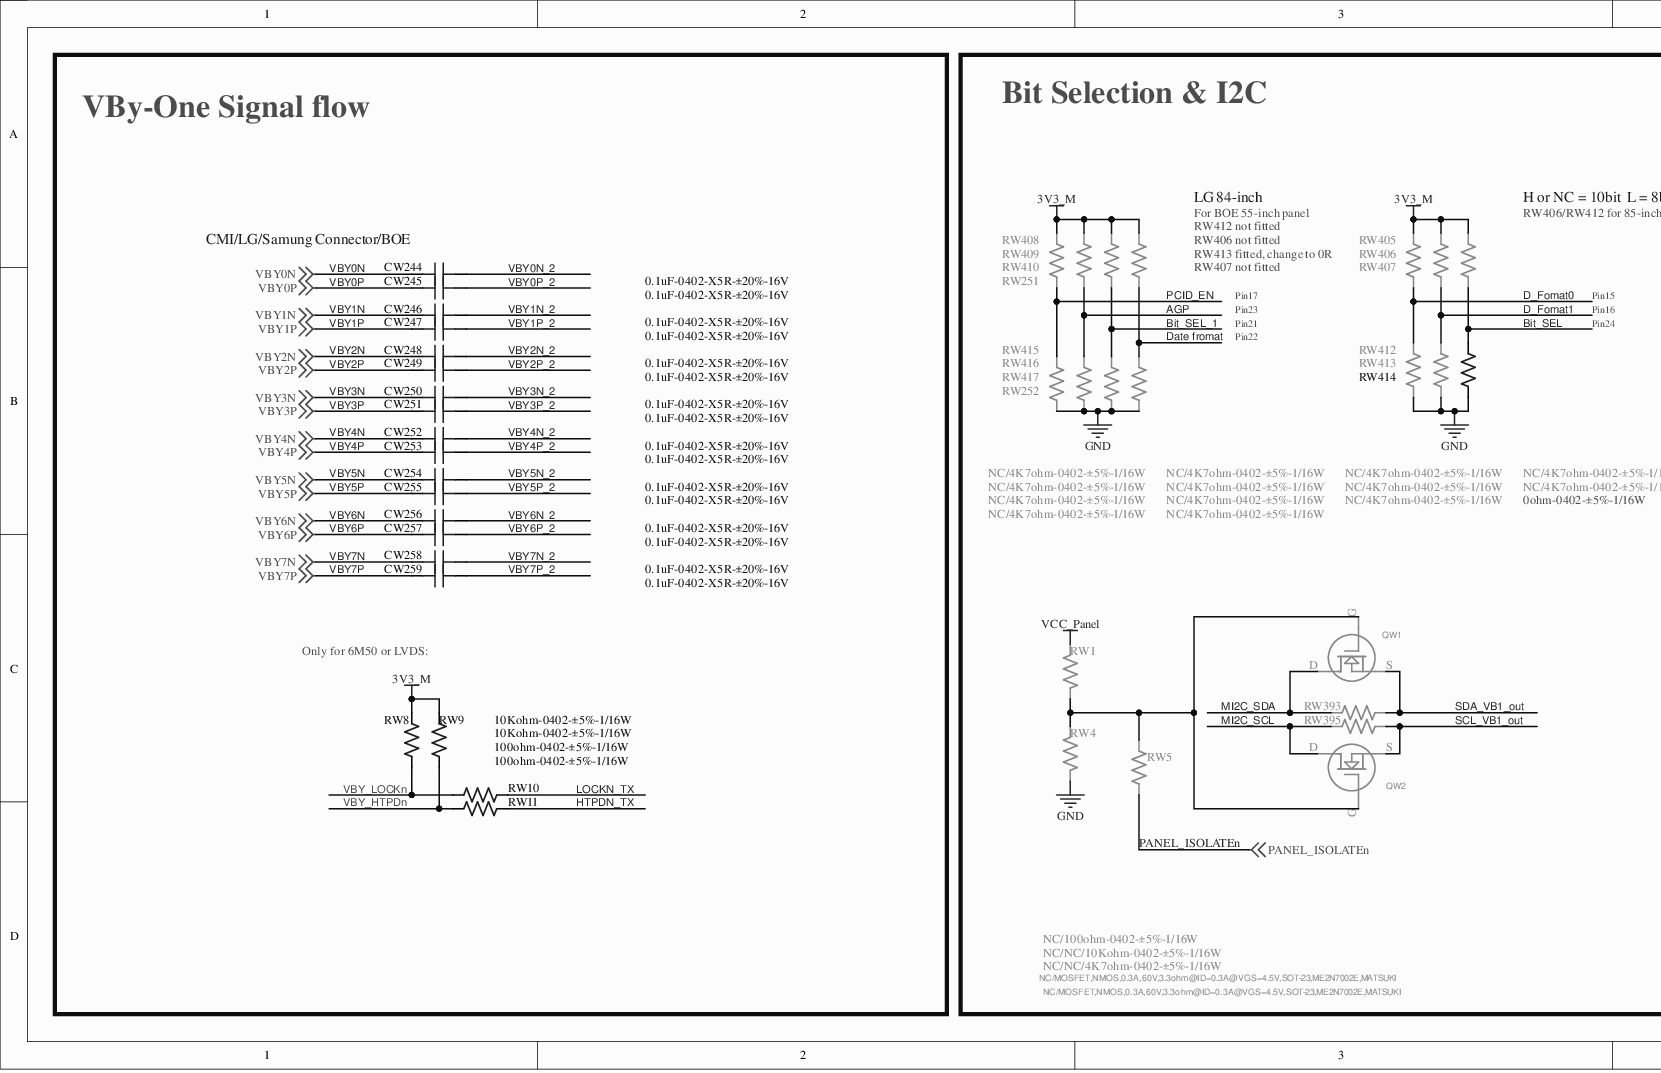
[diagram p0: MISC86290-12.SchDoc, left]
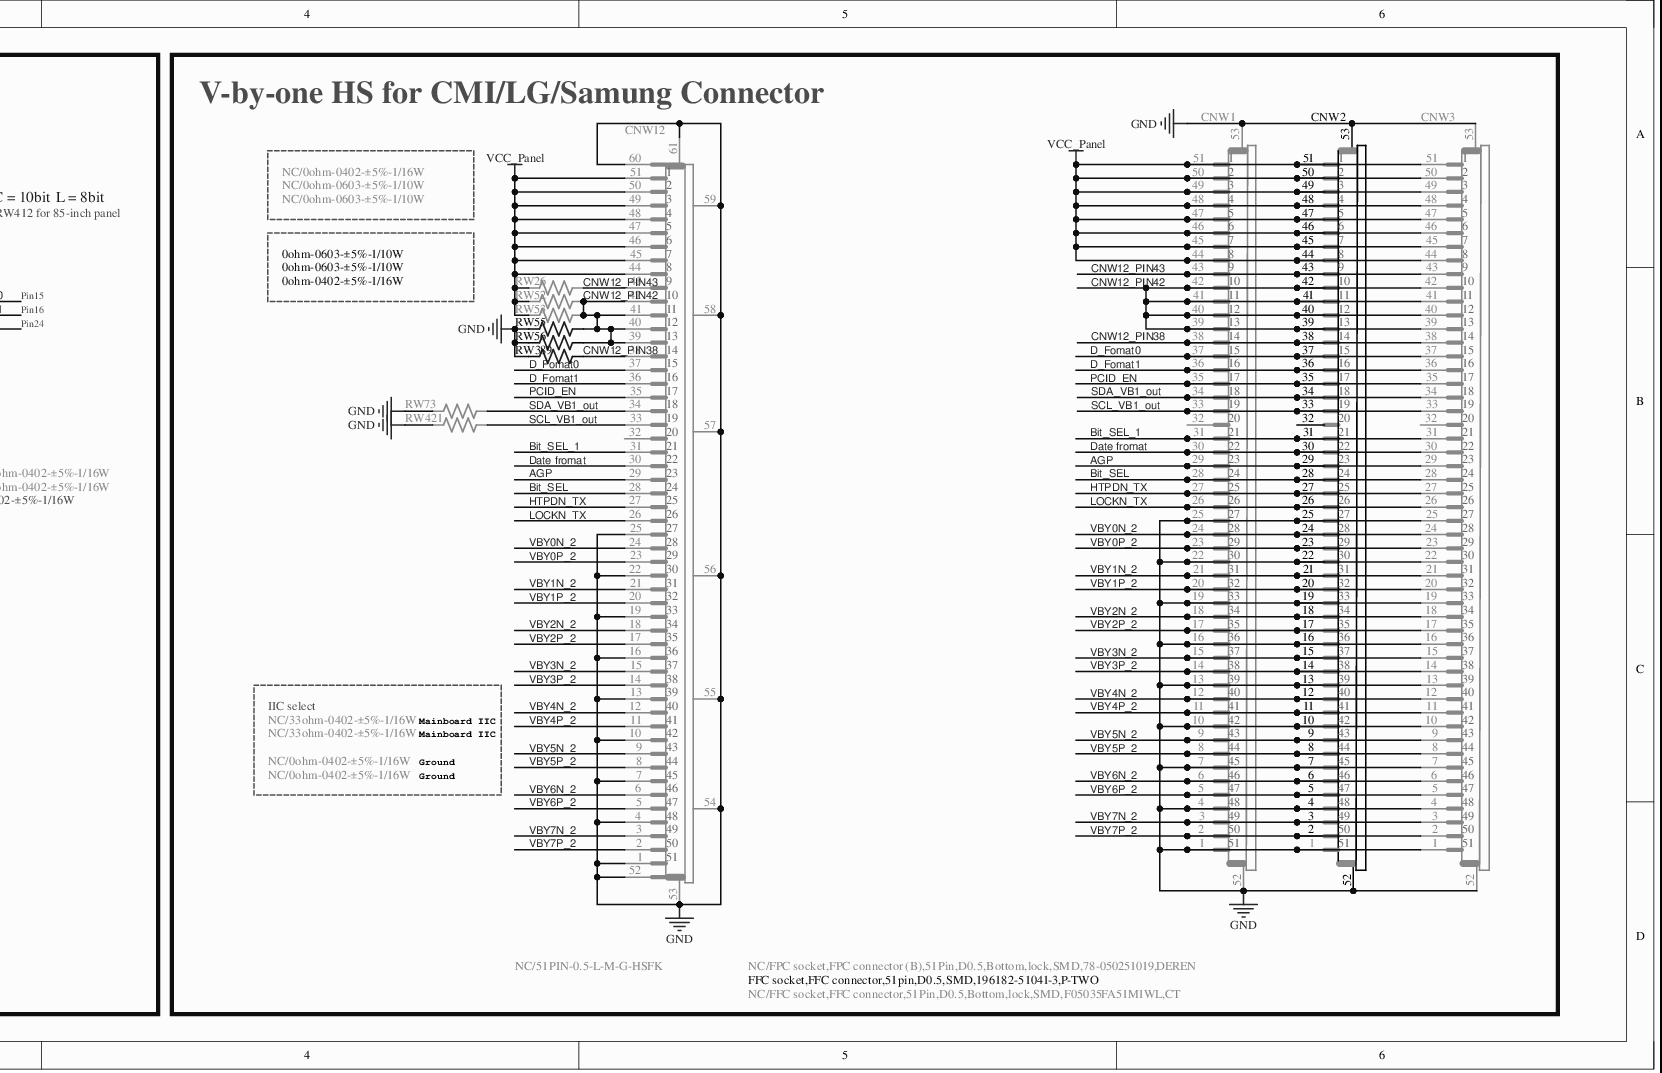
[diagram p1: MISC86290-12.SchDoc, right]
# Altium project MISC86290.PrjPcb (part 9 of 13)

## Sheet MISC86290-12.SchDoc
size 596 x 198 mm

### Parts
CNW1  NC/FPC socket,FPC connector (B),51Pin,D0.5,Bottom,lock,SMD,78-050251019,DEREN  [FFC51H/0.5S-10]
CNW2  FFC socket,FFC connector,51pin,D0.5,SMD,196182-51041-3,P-TWO  [FFC51-H/0.5S-1]
CNW3  NC/FFC socket,FFC connector,51Pin,D0.5,Bottom,lock,SMD,F05035FA51M1WL,CT  [FFC51H/0.5S-12]
CNW12  NC/51PIN-0.5-L-M-G-HSFK  [FFC51H/0.5SA-1]
CW244  0.1uF-0402-X5R-±20%-16V  [C0402]
CW245  0.1uF-0402-X5R-±20%-16V  [C0402]
CW246  0.1uF-0402-X5R-±20%-16V  [C0402]
CW247  0.1uF-0402-X5R-±20%-16V  [C0402]
CW248  0.1uF-0402-X5R-±20%-16V  [C0402]
CW249  0.1uF-0402-X5R-±20%-16V  [C0402]
CW250  0.1uF-0402-X5R-±20%-16V  [C0402]
CW251  0.1uF-0402-X5R-±20%-16V  [C0402]
CW252  0.1uF-0402-X5R-±20%-16V  [C0402]
CW253  0.1uF-0402-X5R-±20%-16V  [C0402]
CW254  0.1uF-0402-X5R-±20%-16V  [C0402]
CW255  0.1uF-0402-X5R-±20%-16V  [C0402]
CW256  0.1uF-0402-X5R-±20%-16V  [C0402]
CW257  0.1uF-0402-X5R-±20%-16V  [C0402]
CW258  0.1uF-0402-X5R-±20%-16V  [C0402]
CW259  0.1uF-0402-X5R-±20%-16V  [C0402]
QW1  NC/MOSFET,NMOS,0.3A,60V,3.3ohm@ID=0.3A@VGS=4.5V,SOT-23,ME2N7002E,MATSUKI  [SOT-23-7]
QW2  NC/MOSFET,NMOS,0.3A,60V,3.3ohm@ID=0.3A@VGS=4.5V,SOT-23,ME2N7002E,MATSUKI  [SOT-23-7]
RW1  NC/NC/10Kohm-0402-±5%-1/16W  [R0402]
RW4  NC/NC/4K7ohm-0402-±5%-1/16W  [R0402]
RW5  NC/100ohm-0402-±5%-1/16W  [R0402]
RW8  10Kohm-0402-±5%-1/16W  [R0402]
RW9  10Kohm-0402-±5%-1/16W  [R0402]
RW10  100ohm-0402-±5%-1/16W  [R0402]
RW11  100ohm-0402-±5%-1/16W  [R0402]
RW26  NC/0ohm-0402-±5%-1/16W  [R0402]
RW52  NC/0ohm-0603-±5%-1/10W  [R0603]
RW53  NC/0ohm-0603-±5%-1/10W  [R0603]
RW55  0ohm-0603-±5%-1/10W  [R0603]
RW56  0ohm-0603-±5%-1/10W  [R0603]
RW73  NC/0ohm-0402-±5%-1/16W  [R0402]
RW251  NC/4K7ohm-0402-±5%-1/16W  [R0402]
RW252  NC/4K7ohm-0402-±5%-1/16W  [R0402]
RW389  0ohm-0402-±5%-1/16W  [R0402]
RW393  NC/33ohm-0402-±5%-1/16W  [R0402]
RW395  NC/33ohm-0402-±5%-1/16W  [R0402]
RW405  NC/4K7ohm-0402-±5%-1/16W  [R0402]
RW406  NC/4K7ohm-0402-±5%-1/16W  [R0402]
RW407  NC/4K7ohm-0402-±5%-1/16W  [R0402]
RW408  NC/4K7ohm-0402-±5%-1/16W  [R0402]
RW409  NC/4K7ohm-0402-±5%-1/16W  [R0402]
RW410  NC/4K7ohm-0402-±5%-1/16W  [R0402]
RW412  NC/4K7ohm-0402-±5%-1/16W  [R0402]
RW413  NC/4K7ohm-0402-±5%-1/16W  [R0402]
RW414  0ohm-0402-±5%-1/16W  [R0402]
RW415  NC/4K7ohm-0402-±5%-1/16W  [R0402]
RW416  NC/4K7ohm-0402-±5%-1/16W  [R0402]
RW417  NC/4K7ohm-0402-±5%-1/16W  [R0402]
RW421  NC/0ohm-0402-±5%-1/16W  [R0402]

### Blocks framed on the sheet
VBy-One Signal flow: CW244-CW259 RW8-RW11
Bit Selection & I2C: QW1 QW2 RW1 RW4 RW5 RW251 RW252 RW393 RW395 RW405-RW410 RW412-RW417
V-by-one HS for CMI/LG/Samung Connector: CNW1-CNW3 CNW12 RW26 RW52 RW53 RW55 RW56 RW73 RW389 RW421

### Nets
3V3_M: RW8.1 RW9.1 RW251.2 RW405.2 RW406.2 RW407.2 RW408.2 RW409.2 RW410.2
GND: CNW1.1 CNW1.4 CNW1.7 CNW1.10 CNW1.13 CNW1.16 CNW1.19 CNW1.22 CNW1.25 CNW1.52 CNW1.53 CNW2.1 CNW2.4 CNW2.7 CNW2.10 CNW2.13 CNW2.16 CNW2.19 CNW2.22 CNW2.25 CNW2.52 CNW2.53 CNW3.1 CNW3.4 CNW3.7 CNW3.10 CNW3.13 CNW3.16 CNW3.19 CNW3.22 CNW3.25 CNW3.52 CNW3.53 CNW12.1 CNW12.4 CNW12.7 CNW12.10 CNW12.13 CNW12.16 CNW12.19 CNW12.22 CNW12.25 CNW12.52 CNW12.53 CNW12.54 CNW12.55 CNW12.56 CNW12.57 CNW12.58 CNW12.59 CNW12.60 CNW12.61 RW4.1 RW55.1 RW56.1 RW73.2 RW252.1 RW389.1 RW412.1 RW413.1 RW414.1 RW415.1 RW416.1 RW417.1 RW421.2
VCC_Panel: CNW1.44 CNW1.45 CNW1.46 CNW1.47 CNW1.48 CNW1.49 CNW1.50 CNW1.51 CNW2.44 CNW2.45 CNW2.46 CNW2.47 CNW2.48 CNW2.49 CNW2.50 CNW2.51 CNW3.44 CNW3.45 CNW3.46 CNW3.47 CNW3.48 CNW3.49 CNW3.50 CNW3.51 CNW12.44 CNW12.45 CNW12.46 CNW12.47 CNW12.48 CNW12.49 CNW12.50 CNW12.51 RW1.2 RW26.2 RW52.1 RW53.1
AGP: CNW1.29 CNW2.29 CNW3.29 CNW12.29 RW409.1 RW416.2
Bit_SEL: CNW1.28 CNW2.28 CNW3.28 CNW12.28 RW407.1 RW414.2
Bit_SEL_1: CNW1.31 CNW2.31 CNW3.31 CNW12.31 RW410.1 RW417.2
CNW12_PIN38: CNW1.38 CNW2.38 CNW3.38 CNW12.38 RW389.2
CNW12_PIN42: CNW1.39 CNW1.40 CNW1.41 CNW1.42 CNW2.39 CNW2.40 CNW2.41 CNW2.42 CNW3.39 CNW3.40 CNW3.41 CNW3.42 CNW12.39 CNW12.40 CNW12.41 CNW12.42 RW52.2 RW53.2 RW55.2 RW56.2
CNW12_PIN43: CNW1.43 CNW2.43 CNW3.43 CNW12.43 RW26.1
D_Fomat0: CNW1.37 CNW2.37 CNW3.37 CNW12.37 RW405.1 RW412.2
D_Fomat1: CNW1.36 CNW2.36 CNW3.36 CNW12.36 RW406.1 RW413.2
Date fromat: CNW1.30 CNW2.30 CNW3.30 CNW12.30 RW251.1 RW252.2
HTPDN_TX: CNW1.27 CNW2.27 CNW3.27 CNW12.27 RW11.1
LOCKN_TX: CNW1.26 CNW2.26 CNW3.26 CNW12.26 RW10.1
MI2C_SCL: QW2.D RW395.2
MI2C_SDA: QW1.D RW393.2
PANEL_ISOLATEn: RW5.1 ; off-sheet PANEL_ISOLATEn
PCID_EN: CNW1.35 CNW2.35 CNW3.35 CNW12.35 RW408.1 RW415.2
SCL_VB1_out: CNW1.33 CNW2.33 CNW3.33 CNW12.33 QW2.S RW395.1 RW421.1
SDA_VB1_out: CNW1.34 CNW2.34 CNW3.34 CNW12.34 QW1.S RW73.1 RW393.1
VBY0N: CW244.1 ; off-sheet VBY0N
VBY0N_2: CNW1.24 CNW2.24 CNW3.24 CNW12.24 CW244.2
VBY0P: CW245.1 ; off-sheet VBY0P
VBY0P_2: CNW1.23 CNW2.23 CNW3.23 CNW12.23 CW245.2
VBY1N: CW246.1 ; off-sheet VBY1N
VBY1N_2: CNW1.21 CNW2.21 CNW3.21 CNW12.21 CW246.2
VBY1P: CW247.1 ; off-sheet VBY1P
VBY1P_2: CNW1.20 CNW2.20 CNW3.20 CNW12.20 CW247.2
VBY2N: CW248.1 ; off-sheet VBY2N
VBY2N_2: CNW1.18 CNW2.18 CNW3.18 CNW12.18 CW248.2
VBY2P: CW249.1 ; off-sheet VBY2P
VBY2P_2: CNW1.17 CNW2.17 CNW3.17 CNW12.17 CW249.2
VBY3N: CW250.1 ; off-sheet VBY3N
VBY3N_2: CNW1.15 CNW2.15 CNW3.15 CNW12.15 CW250.2
VBY3P: CW251.1 ; off-sheet VBY3P
VBY3P_2: CNW1.14 CNW2.14 CNW3.14 CNW12.14 CW251.2
VBY4N: CW252.1 ; off-sheet VBY4N
VBY4N_2: CNW1.12 CNW2.12 CNW3.12 CNW12.12 CW252.2
VBY4P: CW253.1 ; off-sheet VBY4P
VBY4P_2: CNW1.11 CNW2.11 CNW3.11 CNW12.11 CW253.2
VBY5N: CW254.1 ; off-sheet VBY5N
VBY5N_2: CNW1.9 CNW2.9 CNW3.9 CNW12.9 CW254.2
VBY5P: CW255.1 ; off-sheet VBY5P
VBY5P_2: CNW1.8 CNW2.8 CNW3.8 CNW12.8 CW255.2
VBY6N: CW256.1 ; off-sheet VBY6N
VBY6N_2: CNW1.6 CNW2.6 CNW3.6 CNW12.6 CW256.2
VBY6P: CW257.1 ; off-sheet VBY6P
VBY6P_2: CNW1.5 CNW2.5 CNW3.5 CNW12.5 CW257.2
VBY7N: CW258.1 ; off-sheet VBY7N
VBY7N_2: CNW1.3 CNW2.3 CNW3.3 CNW12.3 CW258.2
VBY7P: CW259.1 ; off-sheet VBY7P
VBY7P_2: CNW1.2 CNW2.2 CNW3.2 CNW12.2 CW259.2
VBY_HTPDn: RW9.2 RW11.2
VBY_LOCKn: RW8.2 RW10.2
NetQW1_G: QW1.G QW2.G RW1.1 RW4.2 RW5.2

Not connected (* = marked no-connect by the designer): CNW1 32*; CNW2 32*; CNW3 32*; CNW12 32*

### Notes on the sheet
- LG 84-inch
- H or NC = 10bit  L = 8bit
- (near CNW12) 1
- (near CNW12) 2
- (near CNW12) 3
- (near CNW1) 1
- (near CNW1) 2
- (near CNW1) 3
- (near CNW1) 4
- (near CNW2) 1
- (near CNW2) 2
- (near CNW2) 3
- (near CNW2) 4
- (near CNW3) 1
- (near CNW3) 2
- (near CNW3) 3
- (near CNW3) 4
- CMI/LG/Samung Connector/BOE
- For BOE 55-inch panel
- RW412 not fitted
- RW406 not fitted
- RW413 fitted, change to 0R
- RW407 not fitted
- RW406/RW412 for 85-inch panel
- (near CNW12) 4
- (near CNW12) 5
- (near CNW12) 6
- (near CNW12) 7
- (near CNW12) 8
- (near CNW1) 5
- (near CNW1) 6
- (near CNW1) 7
- (near CNW1) 8
- (near CNW1) 9
- (near CNW2) 5
- (near CNW2) 6
- (near CNW2) 7
- (near CNW2) 8
- (near CNW2) 9
- (near CNW3) 5
- (near CNW3) 6
- (near CNW3) 7
- (near CNW3) 8
- (near CNW3) 9
- Pin17
- Pin21
- Pin22
- Pin23
- Pin15
- Pin16
- Pin24
- (near CNW12) 9
- (near CNW12) 10
- (near CNW12) 11
- (near CNW12) 12
- (near CNW12) 13
- (near CNW1) 10
- (near CNW1) 11
- (near CNW1) 12
- (near CNW1) 13
- (near CNW1) 14
- (near CNW2) 10
- (near CNW2) 11
- (near CNW2) 12
- (near CNW2) 13
- (near CNW2) 14
- (near CNW3) 10
- (near CNW3) 11
- (near CNW3) 12
- (near CNW3) 13
- (near CNW3) 14
- (near CNW12) 14
- (near CNW12) 15
- (near CNW12) 16
- (near CNW12) 17
- (near CNW12) 18
- (near CNW1) 15
- (near CNW1) 16
- (near CNW1) 17
- (near CNW1) 18
- (near CNW1) 19
- (near CNW2) 15
- (near CNW2) 16
- (near CNW2) 17
- (near CNW2) 18
- (near CNW2) 19
- (near CNW3) 15
- (near CNW3) 16
- (near CNW3) 17
- (near CNW3) 18
- (near CNW3) 19
- (near CNW12) 19
- (near CNW12) 20
- (near CNW12) 21
- (near CNW12) 22
- (near CNW12) 23
- (near CNW1) 20
- (near CNW1) 21
- (near CNW1) 22
- (near CNW1) 23
- (near CNW1) 24
- (near CNW2) 20
- (near CNW2) 21
- (near CNW2) 22
- (near CNW2) 23
- (near CNW2) 24
- (near CNW3) 20
- (near CNW3) 21
- (near CNW3) 22
- (near CNW3) 23
- (near CNW3) 24
- (near CNW12) 24
- (near CNW12) 25
- (near CNW12) 26
- (near CNW12) 27
- (near CNW12) 28
- (near CNW1) 25
- (near CNW1) 26
- (near CNW1) 27
- (near CNW1) 28
- (near CNW1) 29
- (near CNW2) 25
- (near CNW2) 26
- (near CNW2) 27
- (near CNW2) 28
- (near CNW2) 29
- (near CNW3) 25
- (near CNW3) 26
- (near CNW3) 27
- (near CNW3) 28
- (near CNW3) 29
- (near CNW12) 29
- (near CNW12) 30
- (near CNW12) 31
- (near CNW12) 32
- (near CNW12) 33
- (near CNW1) 30
- (near CNW1) 31
- (near CNW1) 32
- (near CNW1) 33
- (near CNW1) 34
- (near CNW2) 30
- (near CNW2) 31
- (near CNW2) 32
- (near CNW2) 33
- (near CNW2) 34
- (near CNW3) 30
- (near CNW3) 31
- (near CNW3) 32
- (near CNW3) 33
- (near CNW3) 34
- Only for 6M50 or LVDS:
- (near CNW12) 34
- (near CNW12) 35
- (near CNW12) 36
- (near CNW12) 37
- (near CNW12) 38
- (near CNW1) 35
- (near CNW1) 36
- (near CNW1) 37
- (near CNW1) 38
- (near CNW1) 39
- (near CNW2) 35
- (near CNW2) 36
- (near CNW2) 37
- (near CNW2) 38
- (near CNW2) 39
- (near CNW3) 35
- (near CNW3) 36
- (near CNW3) 37
- (near CNW3) 38
- (near CNW3) 39
- IIC select
- Mainboard IIC
- (near CNW12) 39
- (near CNW12) 40
- (near CNW12) 41
- (near CNW12) 42
- (near CNW12) 43
- (near CNW1) 40
- (near CNW1) 41
- (near CNW1) 42
- (near CNW1) 43
- (near CNW1) 44
- (near CNW2) 40
- (near CNW2) 41
- (near CNW2) 42
- (near CNW2) 43
- (near CNW2) 44
- (near CNW3) 40
- (near CNW3) 41
- (near CNW3) 42
- (near CNW3) 43
- (near CNW3) 44
- Ground
- (near CNW12) 44
- (near CNW12) 45
- (near CNW12) 46
- (near CNW12) 47
- (near CNW12) 48
- (near CNW1) 45
- (near CNW1) 46
- (near CNW1) 47
- (near CNW1) 48
- (near CNW1) 49
- (near CNW2) 45
- (near CNW2) 46
- (near CNW2) 47
- (near CNW2) 48
- (near CNW2) 49
- (near CNW3) 45
- (near CNW3) 46
- (near CNW3) 47
- (near CNW3) 48
- (near CNW3) 49
- (near CNW12) 49
- (near CNW12) 50
- (near CNW12) 51
- (near CNW1) 50
- (near CNW1) 51
- (near CNW2) 50
- (near CNW2) 51
- (near CNW3) 50
- (near CNW3) 51

### Library data of the parts
CNW1 = XXX.XXX.0002122: FPC socket,FPC connector (B),51Pin,D0.5,L,Bottom,lock,SMD,DEREN-D
CNW2 = 51PIN-0.5-L-M-下接-翻盖-H=2.7mm-XFE-D: CN-FFC socket-flip lid
CNW3 = PKG-003664/P000081334: FFC socket,FFC connector,51Pin,D0.5,Bottom,lock,SMD,F05035FA51M1WL,CT-D
CNW12 = FI-RE51S-HF-J-R1500-D: CN-FFC socket-bottom contact
CW244-CW259 = 0.1uF-0402-X5R-±20%-16V-D
QW1 QW2 = 004.007.0000056-D: MOSFET,NMOS,0.3A,60V,3.3ohm@ID=0.3A@VGS=4.5V,SOT-23,ME2N7002E,MATSUKI-D
RW1 RW8 RW9 = 10Kohm-0402-±5%-1/16W-D
RW4 RW251 RW252 RW405-RW410 RW412-RW417 = 4K7ohm-0402-±5%-1/16W-D
RW5 = 100ohm-0402-±5%-1/16W-D
RW10 RW11 RW389 RW393 RW395 = 0ohm-0402-±5%-1/16W-D
RW26 RW73 RW421 = 33ohm-0402-±5%-1/16W-D
RW52 RW53 RW55 RW56 = 0ohm-0603-±5%-1/10W-D

## Sheet MISC86290-13.SchDoc
size 381 x 182 mm
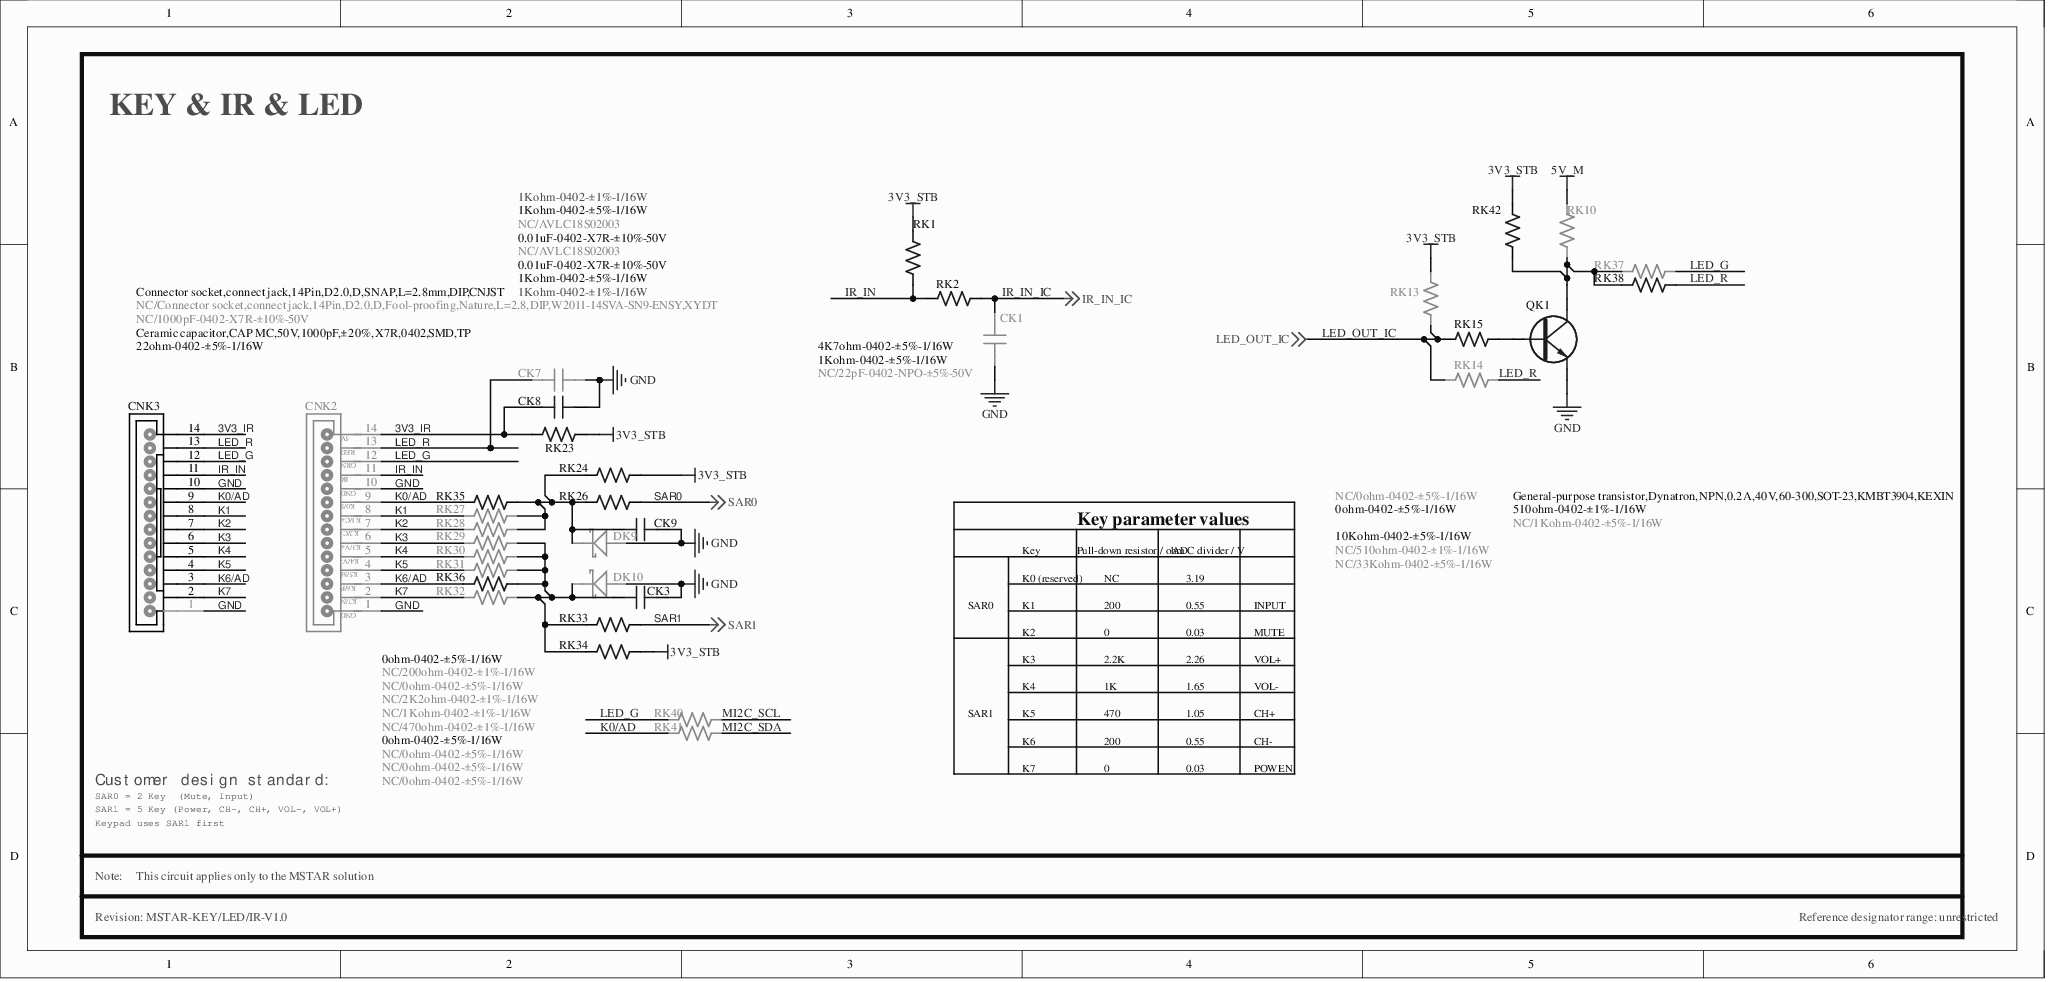
[diagram p2: MISC86290-13.SchDoc]

### Parts
CK1  NC/22pF-0402-NPO-±5%-50V  [C0402]
CK3  0.01uF-0402-X7R-±10%-50V  [C0402]
CK7  NC/1000pF-0402-X7R-±10%-50V  [C0402]
CK8  Ceramic capacitor,CAP MC,50V,1000pF,±20%,X7R,0402,SMD,TP  [C0402]
CK9  0.01uF-0402-X7R-±10%-50V  [C0402]
CNK2  NC/Connector socket,connect jack,14Pin,D2.0,D,Fool-proofing,Nature,L=2.8,DIP,W2011-14SVA-SN9-ENSY,XYDT  [SIP14/2.0D-2]
CNK3  Connector socket,connect jack,14Pin,D2.0,D,SNAP,L=2.8mm,DIP,CNJST  [SIP14/2.0D-5]
DK9  NC/AVLC18S02003  [DIODE-S0402]
DK10  NC/AVLC18S02003  [DIODE-S0402]
QK1  General-purpose transistor,Dynatron,NPN,0.2A,40V,60-300,SOT-23,KMBT3904,KEXIN  [SOT-23]
RK1  4K7ohm-0402-±5%-1/16W  [R0402]
RK2  1Kohm-0402-±5%-1/16W  [R0402]
RK10  NC/1Kohm-0402-±5%-1/16W  [R0402]
RK13  NC/33Kohm-0402-±5%-1/16W  [R0402]
RK14  NC/510ohm-0402-±1%-1/16W  [R0402]
RK15  10Kohm-0402-±5%-1/16W  [R0402]
RK23  22ohm-0402-±5%-1/16W  [R0402]
RK24  1Kohm-0402-±1%-1/16W  [R0402]
RK26  1Kohm-0402-±5%-1/16W  [R0402]
RK27  NC/200ohm-0402-±1%-1/16W  [R0402]
RK28  NC/0ohm-0402-±5%-1/16W  [R0402]
RK29  NC/2K2ohm-0402-±1%-1/16W  [R0402]
RK30  NC/1Kohm-0402-±1%-1/16W  [R0402]
RK31  NC/470ohm-0402-±1%-1/16W  [R0402]
RK32  NC/0ohm-0402-±5%-1/16W  [R0402]
RK33  1Kohm-0402-±5%-1/16W  [R0402]
RK34  1Kohm-0402-±1%-1/16W  [R0402]
RK35  0ohm-0402-±5%-1/16W  [R0402]
RK36  0ohm-0402-±5%-1/16W  [R0402]
RK37  NC/0ohm-0402-±5%-1/16W  [R0402]
RK38  0ohm-0402-±5%-1/16W  [R0402]
RK40  NC/0ohm-0402-±5%-1/16W  [R0402]
RK41  NC/0ohm-0402-±5%-1/16W  [R0402]
RK42  510ohm-0402-±1%-1/16W  [R0402]

### Nets
3V3_STB: RK1.2 RK13.2 RK23.1 RK24.2 RK34.2 RK42.2
5V_M: RK10.2
GND: CK1.1 CK3.1 CK7.1 CK8.1 CK9.1 CNK2.1 CNK2.10 CNK3.1 CNK3.10 DK9.A DK10.A QK1.E
3V3_IR: CK8.2 CNK2.14 CNK3.14 RK23.2
IR_IN: CNK2.11 CNK3.11 RK1.1 RK2.1
IR_IN_IC: CK1.2 RK2.2 ; off-sheet IR_IN_IC
K0/AD: CNK2.9 CNK3.9 RK35.2 RK41.2
K1: CNK2.8 CNK3.8 RK27.2
K2: CNK2.7 CNK3.7 RK28.2
K3: CNK2.6 CNK3.6 RK29.2
K4: CNK2.5 CNK3.5 RK30.1
K5: CNK2.4 CNK3.4 RK31.2
K6/AD: CNK2.3 CNK3.3 RK36.2
K7: CNK2.2 CNK3.2 RK32.2
LED_G: CNK2.12 CNK3.12 RK37.1 RK40.2
LED_OUT_IC: RK13.1 RK14.1 RK15.2 ; off-sheet LED_OUT_IC
LED_R: CK7.2 CNK2.13 CNK3.13 RK14.2 RK38.1
MI2C_SCL: RK40.1
MI2C_SDA: RK41.1
SAR0: RK26.1 ; off-sheet SAR0
SAR1: RK33.1 ; off-sheet SAR1
NetCK3_2: CK3.2 DK10.K RK29.1 RK30.2 RK31.1 RK32.1 RK33.2 RK34.1 RK36.1
NetCK9_2: CK9.2 DK9.K RK24.1 RK26.2 RK27.1 RK28.1 RK35.1
NetQK1_B: QK1.B RK15.1
NetQK1_C: QK1.C RK10.1 RK37.2 RK38.2 RK42.1

### Notes on the sheet
- KEY & IR & LED
- Key parameter values
- Key
- K0 (reserved)
- Pull-down resistor / ohm
- NC
- ADC divider / V
- 3.19
- SAR0
- K1
- K2
- K3
- 200
- 0
- 2.2K
- 0.55
- 0.03
- 2.26
- INPUT
- MUTE
- VOL+
- SAR1
- K4
- K5
- 1K
- 470
- 1.65
- 1.05
- VOL-
- CH+
- Customer design standard:
- SAR0 = 2 Key  (Mute, Input)
- K6
- K7
- CH-
- POWEN
- Keypad uses SAR1 first
- SAR1 = 5 Key (Power, CH-, CH+, VOL-, VOL+)
- Note:
- Revision: MSTAR-KEY/LED/IR-V1.0
- This circuit applies only to the MSTAR solution
- Reference designator range: unrestricted

### Library data of the parts
CK1 = 22pF-0402-NPO-±5%-50V-D
CK3 CK9 = 0.01uF-0402-X7R-±10%-50V-D
CK7 CK8 = 1000pF-0402-X7R-±10%-50V-D
CNK2 = 14PIN-2.0-D-H-G-DHMI-IR&KEY
CNK3 = 14PIN-2.0-D-H-G-带扣-J-DHMI
DK9 DK10 = AVLC18S02003-D
QK1 = LMBT3904LT1G-D-NPN: Q-NPN-#-#-#
RK1 RK28 RK30 = 4K7ohm-0402-±5%-1/16W-D
RK2 RK10 RK26 RK33 RK42 = 1Kohm-0402-±5%-1/16W-D
RK13 = 33Kohm-0402-±5%-1/16W-D
RK14 = 510ohm-0402-±5%-1/16W-D
RK15 = 10Kohm-0402-±5%-1/16W-D
RK23 = 22ohm-0402-±5%-1/16W-D
RK24 RK34 = 4K7ohm-0402-±1%-1/16W-D
RK27 RK32 RK35-RK38 RK40 RK41 = 1K5ohm-0402-±5%-1/16W-D
RK29 RK31 = 12Kohm-0402-±1%-1/16W-D